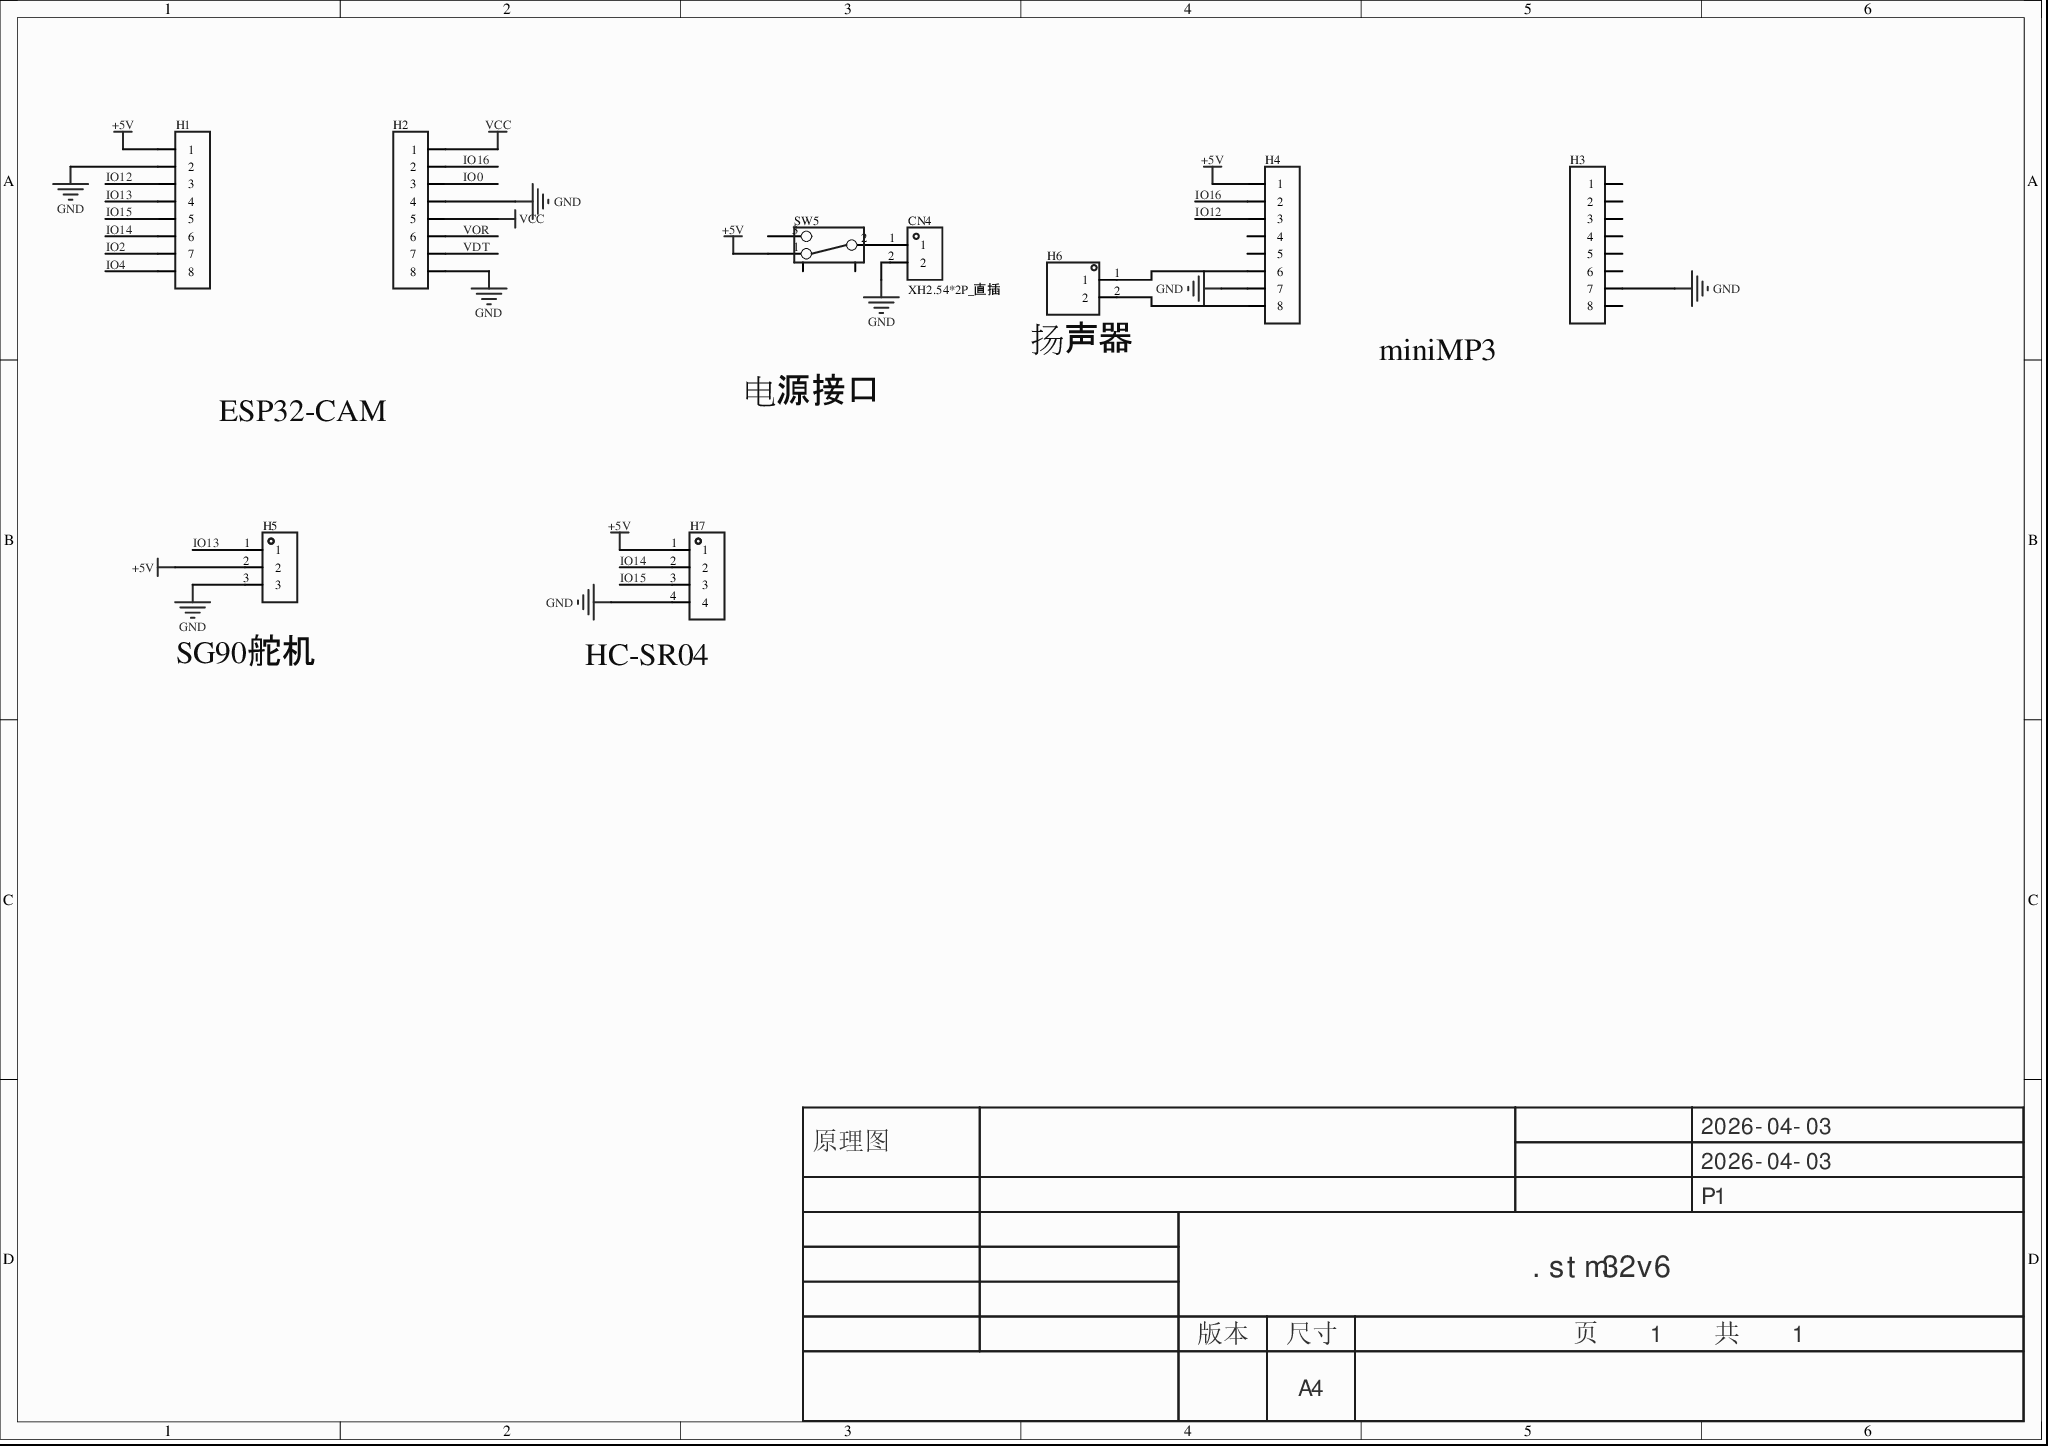
[diagram p0: MISC51682-3.schdoc]
# Altium project MISC51682-2.PrjPcb
1 sheet, 9 parts. Net scope: global (net labels, ports and power ports of the same name join across sheets).
Board file: MISC51682.pcbdoc

## Sheet MISC51682-3.schdoc
size 297 x 209 mm; Version: V1.0; @Project Name: MISC51682; @Page Count: 1; @Update Date: 2026-04-03; @Create Date: 2026-04-03; @Schematic Name: MISC51682; @Page No: 1; @Create Time: 23:22:16; @Update Time: 17:32:40; @Board Name: MISC51682

### Parts
CN4  XH2.54*2P_直插  [CONN-TH_2P-P2.50-XH2.54-2P]
H1  (no value)  [HDR-TH_8P-P2.54-V-F-1]
H2  (no value)  [HDR-TH_8P-P2.54-V-F-1]
H3  (no value)  [HDR-TH_8P-P2.54-V-F-1]
H4  (no value)  [HDR-TH_8P-P2.54-V-F-1]
H5  (no value)  [HDR-TH_3P-P2.54-V-F]
H6  (no value)  [HDR-TH_2P-P2.54-V-M-1]
H7  (no value)  [HDR-TH_4P-P2.54-V-F]
SW5  (no value)  [拨动开关]

### Nets
+5V: H1.1 H4.1 H5.2 H7.1 SW5.1
GND: CN4.2 H1.2 H2.4 H2.8 H3.7 H4.7 H5.3 H7.4
VCC: H2.1 H2.5
IO0: H2.3
IO2: H1.7
IO4: H1.8
IO12: H1.3 H4.3
IO13: H1.4 H5.1
IO14: H1.6 H7.2
IO15: H1.5 H7.3
IO16: H2.2 H4.2
VDT: H2.7
VOR: H2.6
NetCN4_1: CN4.1 SW5.2
NetH4_6: H4.6 H6.1
NetH4_8: H4.8 H6.2

Not connected (* = marked no-connect by the designer): H3 1 2 3 4 5 6 8; H4 4 5; SW5 3 4 5

### Notes on the sheet
- ESP32-CAM
- 电源接口
- (near H6) 扬声器
- miniMP3
- (near H5) SG90舵机
- (near H7) HC-SR04
- 2026-04-03
- 原理图
- P1
- .stm32v6
- 版本
- 尺寸
- A4
- 页    1    共    1

### Library data of the parts
CN4 = XH2.54*2P_直插: 3D Model: 325c595e30db4df8abe76612dd40b0fa0819f05c4eef4c71ace90d822a990e87; 3D Model Transform: 295.275,228.346,0,180,0,0,-0.002,-20.079,-137.795; AddInBom: yes; Symbol: XH2.54*2P_直插; Device: XH2.54*2P_直插; LCSC Part Name: XH2.54*2P_直插; Supplier Part: C9900008615; Manufacturer Part: XH2.54*2P_直插; Supplier Footprint: XH2.54_2P; JLCPCB Part Class: Extended Part; Supplier: LCSC; ConvertToPcb: yes; FootprintName: CONN-TH_2P-P2.50-XH2.54-2P; ModelName: CONN-TH_2P-P2.50-XH2.54-2P
H1-H4 = HDR-F_2.54_1x8P: Symbol: Header-Female-2.54_1x8; AddInBom: yes; ModelId: 0f7e4d9227ef4fa08d5469c22cc70cdb; ModelName: HDR-F-2.54_1x8; ModelTransform: 799.99844,100,0,0,0,0,0,0,-118.11; Device: HDR-F_2.54_1x8P; ConvertToPcb: yes; FootprintName: HDR-TH_8P-P2.54-V-F-1; SupplierPart: C27438; Supplier Footprint: 插件
H5 = HDR-F_2.54_1x3P: Symbol: PM254V-11-03-H85; 3D Model: f3b3cc5aae9641bf9e56fc160cef875b; 3D Model Transform: 299.9994,100,0,0,0,0,0,0,-118.11; ConvertToPcb: yes; ModelName: HDR2.54-F-LI-1X3P; Device: HDR-F_2.54_1x3P; Supplier Part: C541850; Supplier Footprint: 插件; AddInBom: yes; FootprintName: HDR-TH_3P-P2.54-V-F
H6 = HDR-M_2.54_1x2P: Symbol: 210S-1*2P L=11.6MMGold-plated black; ConvertToPcb: yes; ModelId: 79b2e9f2d70a4d68a1b7098f27c6d4c50819f05c4eef4c71ace90d822a990e87; ModelName: HDR-M-2.54_1x2; ModelTransform: 200,100,0,0,0,0,0,0,-118.11; Device: HDR-M_2.54_1x2P; AddInBom: yes; SupplierPart: C124375; Supplier Footprint: 插件; FootprintName: HDR-TH_2P-P2.54-V-M-1
H7 = HDR-F_2.54_1x4P: Symbol: 2.54-1*4P母; 3D Model: d187812051054f85879fcaa51a310d8e0819f05c4eef4c71ace90d822a990e87; 3D Model Transform: 419.6842,98.464,0,0,0,0,0,0,-118.11; ConvertToPcb: yes; Device: HDR-F_2.54_1x4P; Supplier Part: C2718488; Supplier Footprint: 插件; AddInBom: yes; FootprintName: HDR-TH_4P-P2.54-V-F; ModelName: HDR-TH_4P-P2.54-V-F
SW5 = 拨动开关_正: ConvertToPcb: yes; ModelId: 4321fe59a4074cbfb4989553f297c68f0819f05c4eef4c71ace90d822a990e87; ModelName: SW-TH_SS-12D02-VG4; ModelTransform: 370.09,208.7,472.35,0,0,0,0,0,-110; Symbol: 拨动开关; Device: 拨动开关_正; AddInBom: yes; Supplier Footprint: 插件; FootprintName: 拨动开关